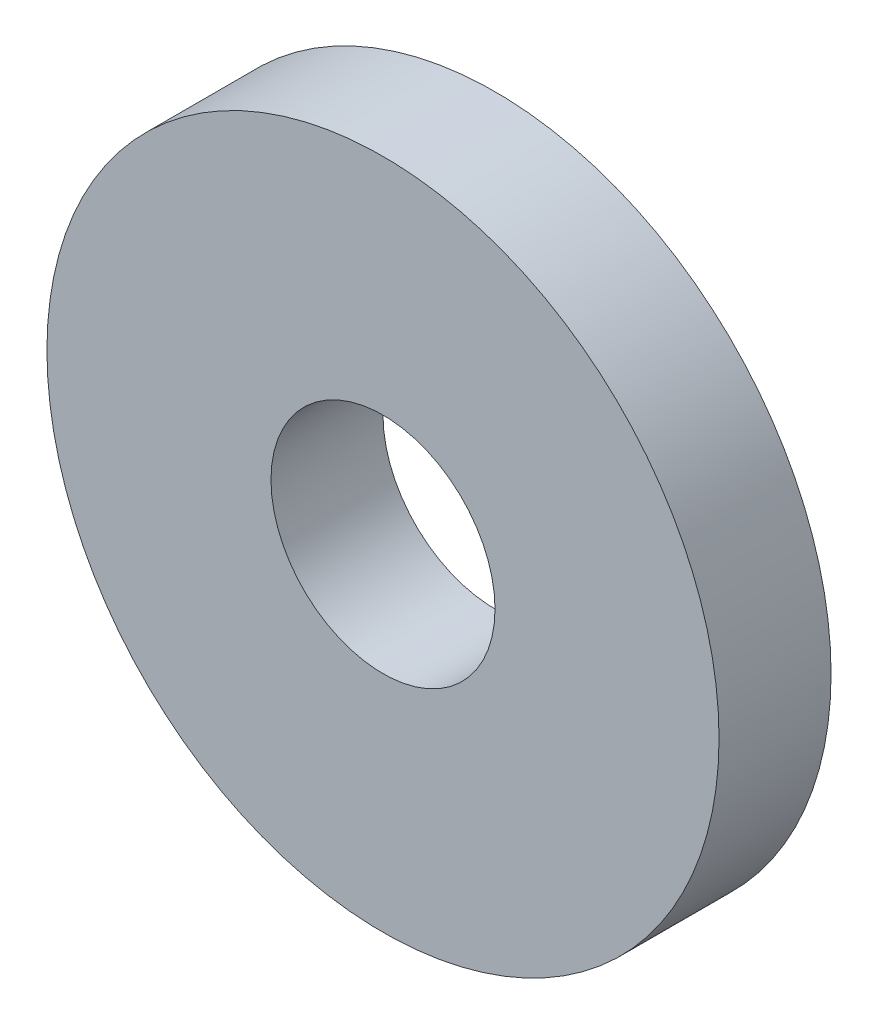
from build123d import *

# Parameters (mm, degrees)
SKETCH_1_R      = 6
SKETCH_1_R_2    = 2
EXTRUDE_1_DEPTH = 2


with BuildPart() as part:
    # 草图1 → 凸台-拉伸1 (new body)
    with BuildSketch(Plane.XY):
        Circle(SKETCH_1_R)
        Circle(SKETCH_1_R_2, mode=Mode.SUBTRACT)
    extrude(amount=EXTRUDE_1_DEPTH)


solid = part.part
